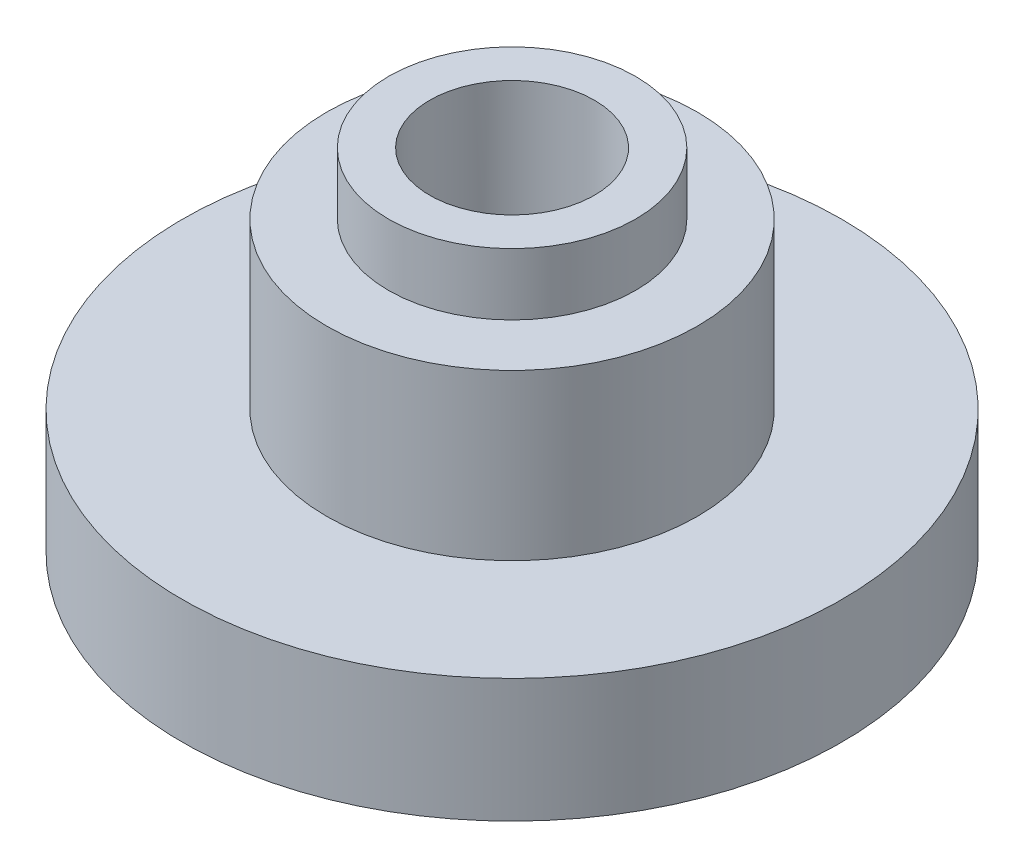
SolidWorks part; units mm, degrees
ref_plane "前视基准面" through (0, 0, 0) normal (0, 0, 1) x (1, 0, 0)
ref_plane "上视基准面" through (0, 0, 0) normal (0, 1, 0) x (1, 0, 0)
ref_plane "右视基准面" through (0, 0, 0) normal (1, 0, 0) x (0, 0, -1)
sketch "草图1" plane through (0, 0, 0) normal (0, 0, 1) x (1, 0, 0)
  line L0 (0, 0) -> (0, 10998.4867) construction
  line L2 (6, 3.6936) -> (6, 0.6936)
  line L3 (6, 0.6936) -> (9, 0.6936)
  line L4 (9, 0.6936) -> (9, -7.3064)
  line L5 (9, -7.3064) -> (16, -7.3064)
  line L6 (16, -7.3064) -> (16, -13.3064)
  line L7 (16, -13.3064) -> (0, -13.3064)
  line L8 (0, -13.3064) -> (0, -9.3064)
  line L11 (6, 3.6936) -> (4, 3.6936)
  line L12 (4, 3.6936) -> (4, -9.3064)
  line L13 (4, -9.3064) -> (0, -9.3064)
  dimension "D1" = 16
  dimension "D2" = 4
  dimension "D3" = 6
  dimension "D4" = 7
  dimension "D5" = 8
  dimension "D6" = 3
  dimension "D7" = 3
  dimension "D8" = 2
revolve "旋转1" add sketch "草图1" angle 360 about L0
sketch "草图2" plane through (0, 0, 0) normal (1, 0, 0) x (0, 0, -1)
  line L0 (16, -7.3064) -> (-16, -7.3064) construction
  circle A0 centre (0, -3.3064) radius 2
  dimension "D2" = 4
  dimension "D1" = 4
extrude "切除-拉伸1" cut sketch "草图2" against normal blind 10
